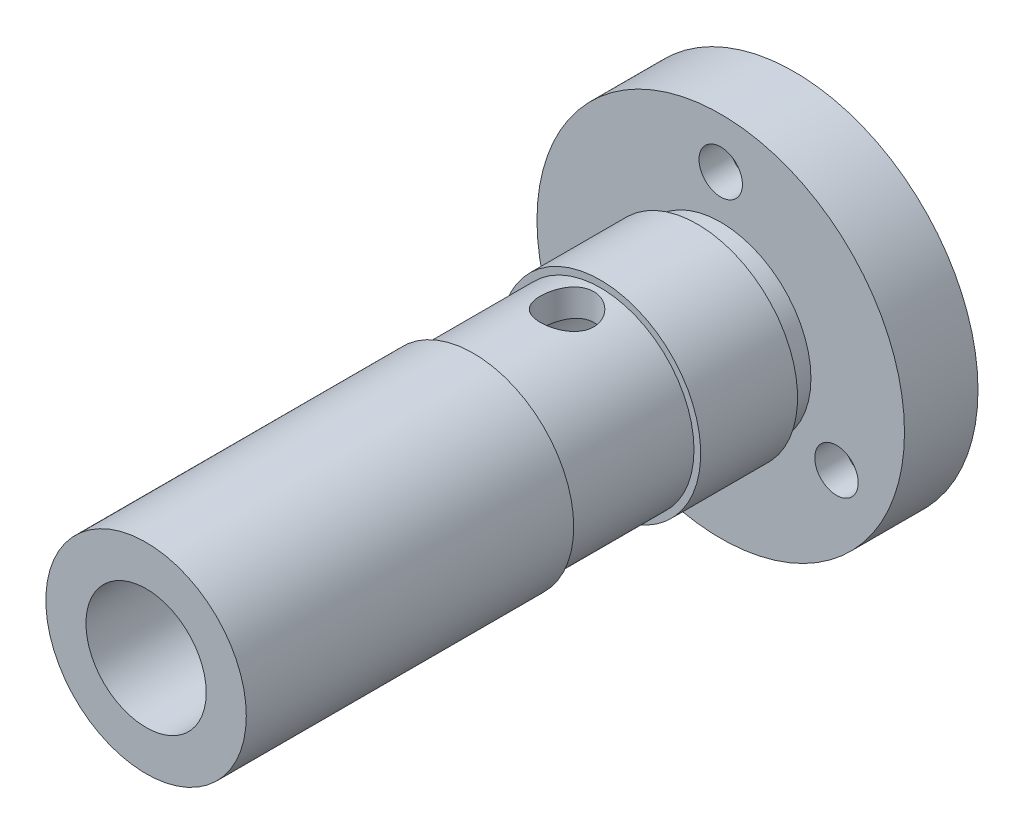
from build123d import *

# Parameters (mm, degrees)
SKETCH1_R           = 27.5
BOSS_EXTRUDE1_DEPTH = 11
SKETCH2_R           = 13.5
BOSS_EXTRUDE2_DEPTH = 3.5
SKETCH3_R           = 15
BOSS_EXTRUDE3_DEPTH = 14.5
SKETCH4_R           = 14
BOSS_EXTRUDE4_DEPTH = 19
SKETCH5_R           = 15
BOSS_EXTRUDE5_DEPTH = 49
SKETCH6_R           = 9
CUT_EXTRUDE1_DEPTH  = 52
SKETCH7_R           = 10
CUT_EXTRUDE2_DEPTH  = 38
SKETCH8_R           = 5.5
CUT_EXTRUDE3_DEPTH  = 6.5
SKETCH9_R           = 3.25
CUT_EXTRUDE4_DEPTH  = 6.5
CIRPATTERN1_COUNT   = 3
SKETCH10_R          = 4
CUT_EXTRUDE5_DEPTH  = 26.75


with BuildPart() as part:
    # Sketch1 → Boss-Extrude1 (new body)
    with BuildSketch(Plane.XY):
        Circle(SKETCH1_R)
    extrude(amount=BOSS_EXTRUDE1_DEPTH)

    # Sketch2 → Boss-Extrude2 (add)
    with BuildSketch(Plane.XY.offset(11)):
        Circle(SKETCH2_R)
    extrude(amount=BOSS_EXTRUDE2_DEPTH)

    # Sketch3 → Boss-Extrude3 (add)
    with BuildSketch(Plane.XY.offset(14.5)):
        with Locations(Location((0, 0, 0), (0, 0, 180))):
            Circle(SKETCH3_R)
    extrude(amount=BOSS_EXTRUDE3_DEPTH)

    # Sketch4 → Boss-Extrude4 (add)
    with BuildSketch(Plane.XY.offset(29)):
        Circle(SKETCH4_R)
    extrude(amount=BOSS_EXTRUDE4_DEPTH)

    # Sketch5 → Boss-Extrude5 (add)
    with BuildSketch(Plane.XY.offset(48)):
        with Locations(Location((0, 0, 0), (0, 0, 180))):
            Circle(SKETCH5_R)
    extrude(amount=BOSS_EXTRUDE5_DEPTH)

    # Sketch6 → Cut-Extrude1 (cut)
    with BuildSketch(Plane.XY.offset(97)):
        Circle(SKETCH6_R)
    extrude(amount=-CUT_EXTRUDE1_DEPTH, mode=Mode.SUBTRACT)

    # Sketch7 → Cut-Extrude2 (cut)
    with BuildSketch(Plane.XY.offset(45)):
        Circle(SKETCH7_R)
    extrude(amount=-CUT_EXTRUDE2_DEPTH, mode=Mode.SUBTRACT)

    # Sketch8 → Cut-Extrude3 (cut)
    with BuildSketch(Plane(origin=(0, 0, 0), x_dir=(-1, 0, 0), z_dir=(0, 0, -1))):
        with Locations((0, 20)):
            Circle(SKETCH8_R)
    cut_extrude3 = extrude(amount=-CUT_EXTRUDE3_DEPTH, mode=Mode.SUBTRACT)

    # Sketch9 → Cut-Extrude4 (cut)
    with BuildSketch(Plane(origin=(0, 0, 6.5), x_dir=(-1, 0, 0), z_dir=(0, 0, -1))):
        with Locations((0, 20)):
            Circle(SKETCH9_R)
    cut_extrude4 = extrude(amount=-CUT_EXTRUDE4_DEPTH, mode=Mode.SUBTRACT)

    # CirPattern1: Cut-Extrude3, Cut-Extrude4 ×3 about axis
    cirpattern1_axis = Axis((0, 0, 0), (0, 0, 1))
    add([cut_extrude3.rotate(cirpattern1_axis, i * 360 / CIRPATTERN1_COUNT) for i in range(1, CIRPATTERN1_COUNT)], mode=Mode.SUBTRACT)
    add([cut_extrude4.rotate(cirpattern1_axis, i * 360 / CIRPATTERN1_COUNT) for i in range(1, CIRPATTERN1_COUNT)], mode=Mode.SUBTRACT)

    # Sketch10 → Cut-Extrude5 (cut, symmetric)
    with BuildSketch(Plane(origin=(0, 0, 0), x_dir=(1, 0, 0), z_dir=(0, 1, 0))):
        with Locations(Location((0, -34, 0), (0, 0, 270))):
            Circle(SKETCH10_R)
    extrude(amount=CUT_EXTRUDE5_DEPTH, both=True, mode=Mode.SUBTRACT)


solid = part.part
